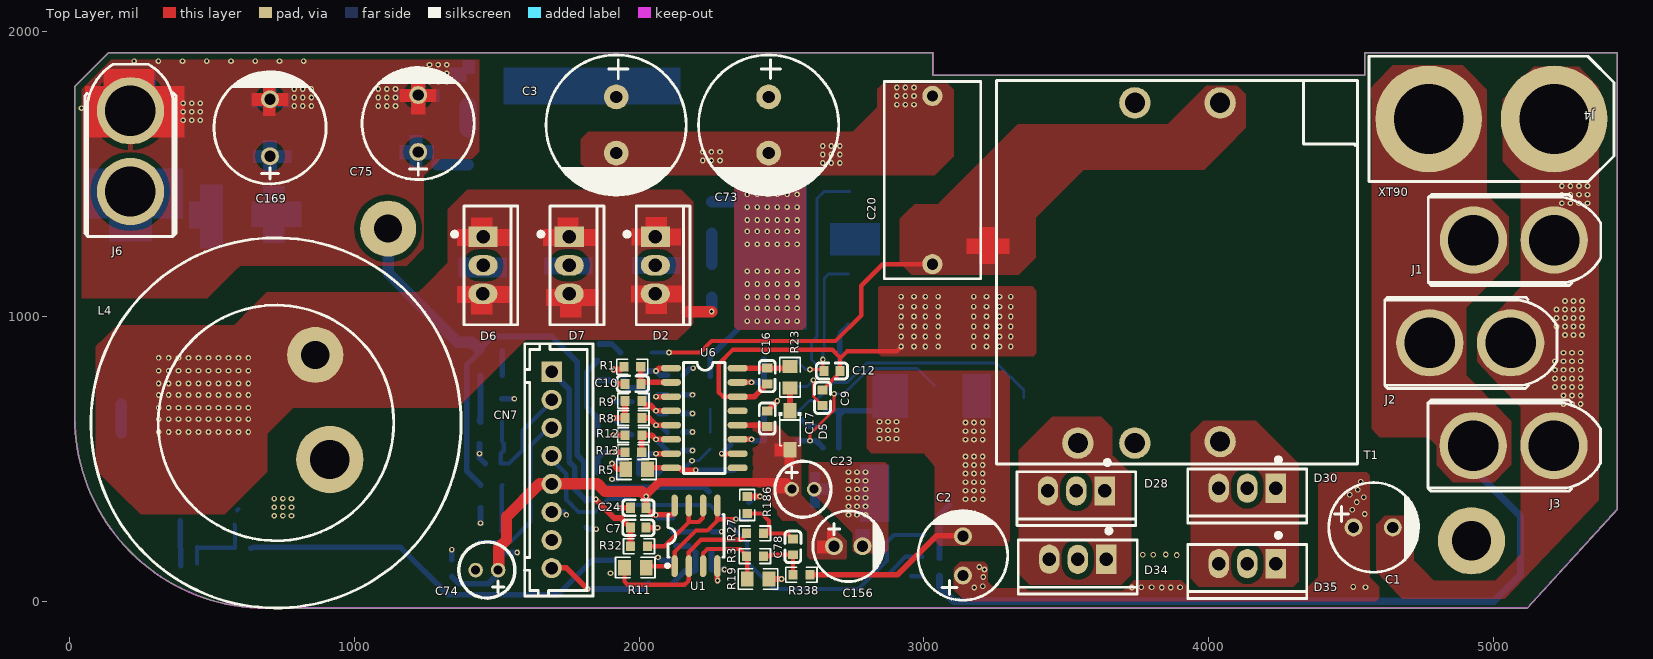
[diagram p0: Top Layer view]
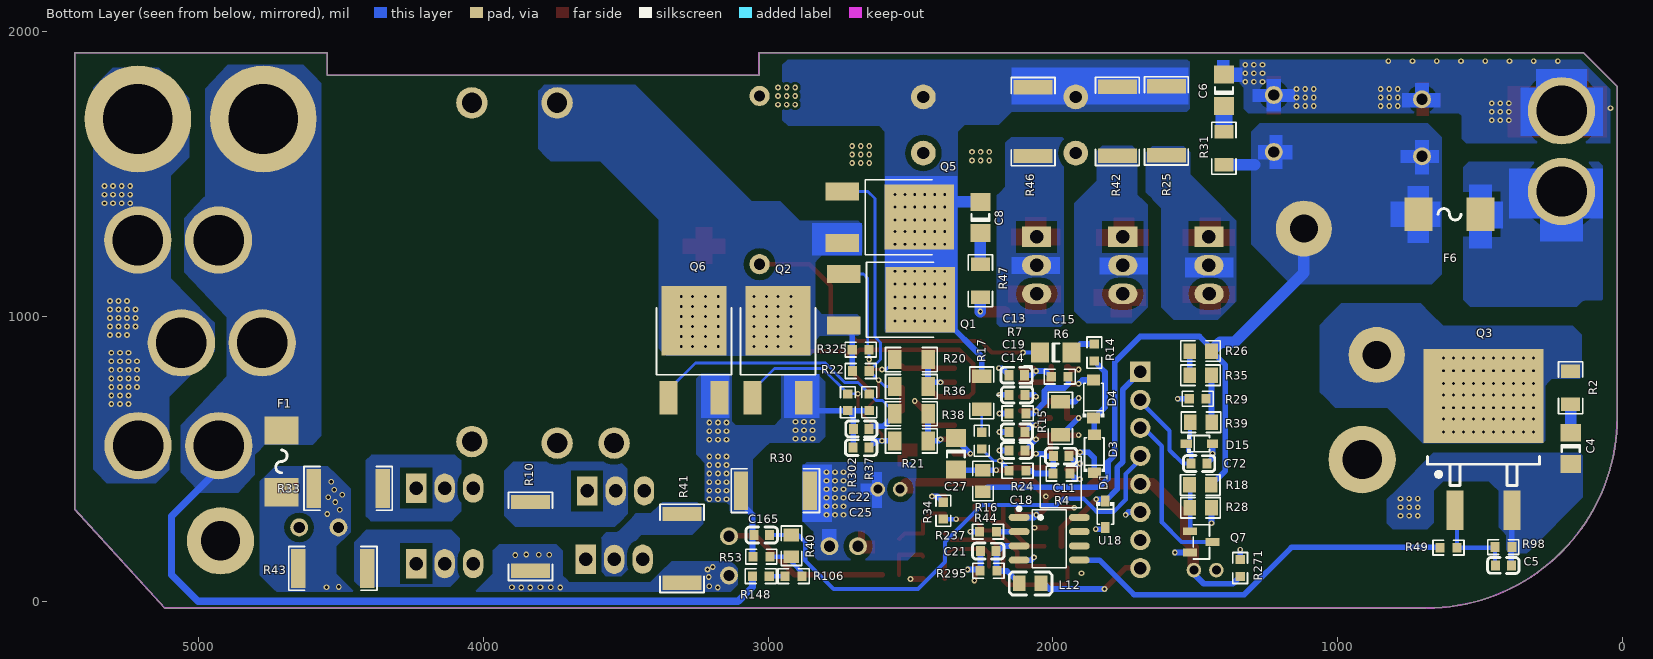
[diagram p1: Bottom Layer view, seen from below]
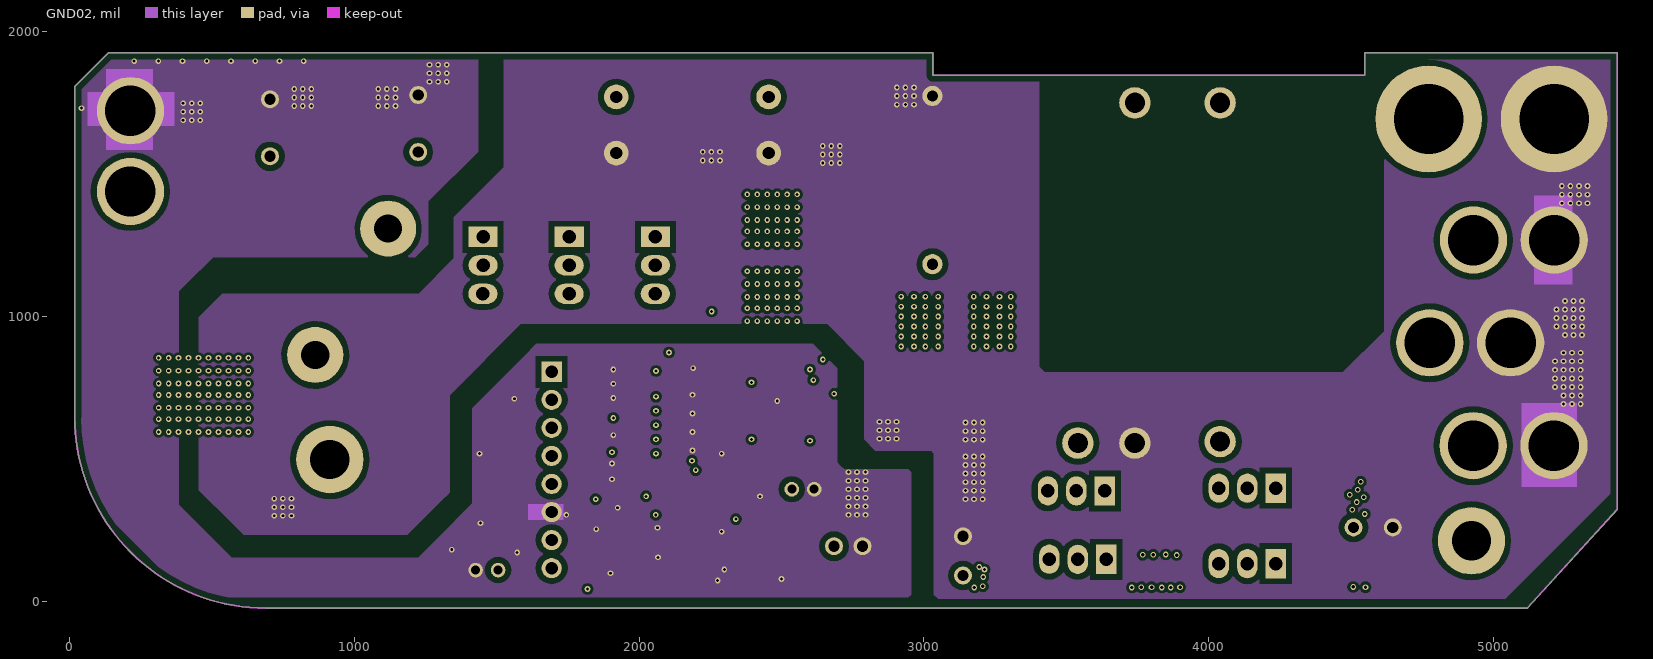
[diagram p2: GND02]
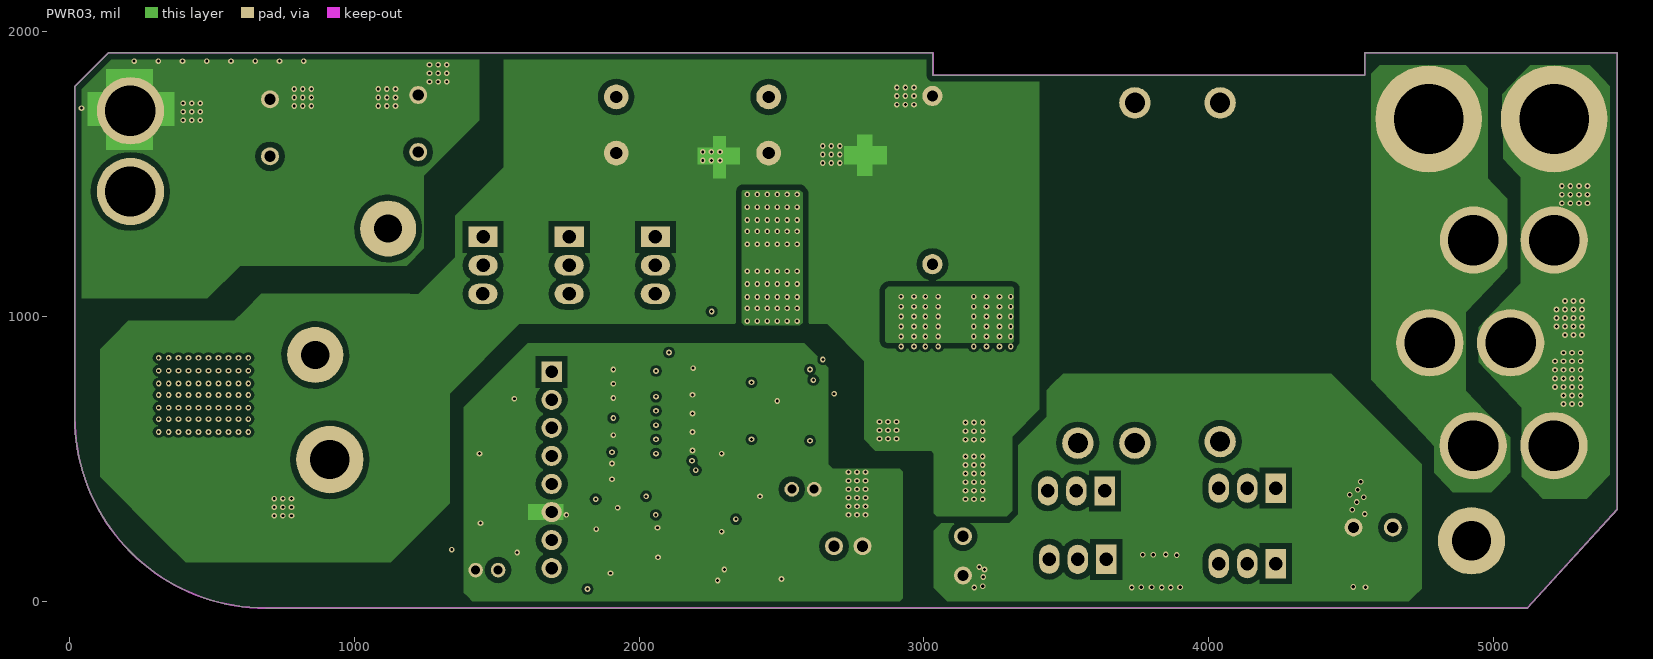
[diagram p3: PWR03]
# Altium PCB MISC84449.PcbDoc (part 1 of 3)
Units mil, origin at the board's own origin, x right, y up, seen from the top; angles counter-clockwise.
Board outline 5413.39 x 1948.82 mil, 4 copper layers (Top Layer, GND02, PWR03, Bottom Layer); 124 components, 66 nets, 298 pads, 442 vias.

## Layer stack, top to bottom (the 12.6 mil dielectric is the usual default, probably not edited)
Top Layer: signal copper 1.4
Dielectric: core 12.6, FR-4, Dk 4.8
GND02: signal copper 1.4
Dielectric: prepreg 12.6, FR-4, Dk 4.8
PWR03: signal copper 1.4
Dielectric: core 12.6, FR-4, Dk 4.8
Bottom Layer: signal copper 1.4

## Board outline
689.14,-22.12 cw(c689.14,647.18) 19.85,647.18 19.85,1808.59 137.96,1926.7 3031.66,1926.7 3031.66,1847.96 4547,1847.96 4547,1926.7 5433.24,1926.7 5433.24,324.34 5118.28,-22.12

## Design rules (kind name [scope] priority, off if disabled: settings)
Clearance 40 [InNetClass('40')] p1 off: gap=30
Clearance Clearance_via [isvia vs inpoly] p2: gap=10
Clearance [InPolygon] p3: gap=20
Clearance all [All] p4: gap=8
ComponentClearance [All] p1 off: gap=10 collisioncheckmode=3 verticalgap=10 showdistances=FALSE
FabricationTestPointUsage TestPointUsage [All] p1: valid=0 allowmultiple=FALSE
FabricationTestpoint Testpoint [(IsPad And (OnTopLayer Or OnBottomLayer))] p1: side=3 testpointundercomponent=TRUE minsize=40 maxsize=100 preferedsize=60 minholesize=0 maxholesize=40 preferedholesize=32 testpointgrid=1 allowsidetop=TRUE allowsidebottom=TRUE usegrid=TRUE gridtolerance=0.01
Height [All] p1 off: minheight=0 maxheight=1000 prefheight=500
HoleSize [All] p1 off: absolutevalues=TRUE maxlimit=100 minlimit=1 maxpercent=80.000 minpercent=20.000
HoleToHoleClearance [All] p1 off: gap=10 allowstackedmicrovias=TRUE
LayerPairs [All] p1 off: enforce=TRUE
MinimumSolderMaskSliver [All] p1 off: minsoldermaskwidth=10
NetAntennae [All] p1: netantennaetolerance=1
PlaneClearance [All] p1: clearance=12
PlaneConnect [All] p1: planeconnectstyle=Relief reliefexpansion=8 reliefentries=4 reliefconductorwidth=10 reliefairgap=10
PolygonConnect PolygonConnect_1 [ISVIA] p1: connectstyle=Direct reliefconductorwidth=10 reliefentries=4 polygonreliefangle="90 Angle"
PolygonConnect [All] p2: connectstyle=Direct reliefconductorwidth=35 reliefentries=4 polygonreliefangle="90 Angle"
RoutingVias [All] p1: holewidth=10 width=20 viastyle="Through Hole" minholewidth=10 minwidth=20 maxholewidth=12 maxwidth=20
SilkToSilkClearance [All] p1 off: silktosilkclearance=10
SilkscreenOverComponentPads [IsPad] p1 off: minsilkscreentomaskgap=10
SolderMaskExpansion [All] p1: expansion=2.5
Width [All] p1: maxlimit=500 minlimit=10 preferedwidth=10
15 further rules are at their usual default settings.

## Components (designator, comment, footprint, x,y, rotation, side; value= is the part's Value field where it differs from the comment)
C1 "390uF" CAP-TH_BD8.0-P3.50-D0.6-FD 4577.65,261.02 r0 top
C2 "390uF" CAP-TH_BD8.0-P3.50-D0.6-FD 3136.98,161.85 r90 top
C3 "560uF" CAP-TH_BD12.5-P5.00-D0.6-FD 1919.99,1673.43 r270 top
C4 "2.2nF" C1206 183,538.12 r270 bottom
C5 "2.2nF" C0603 419.08,127.64 r180 bottom
C6 "2.2nF" C1206 1400,1795.12 r90 bottom
C7 "1nF" C0603 1997.44,260 r180 top
C8 "2.2nF" C1206 2255,1348.68 r90 bottom
C9 "2.2nF" C0603 2644.36,715.92 r90 top
C10 "220nF" C0603 1978.64,765 r0 top
C11 "1uF" C0603 1971.32,511.12 r180 bottom
C12 "2.2nF" C0603 2677.64,810.08 r0 top
C13 "2.2uF" C0603 2127.44,795 r180 bottom
C14 "1nF" C0603 2126.32,596.12 r180 bottom
C15 "NC" C1206 1990,875 r180 bottom
C16 "100nF" C0603 2450,792.44 r90 top
C17 "100nF" C0603 2450,642.56 r270 top
C18 "470pF" C0603 2126.32,531.12 r180 bottom
C19 "1nF" C0603 2126.32,726.12 r0 bottom
C20 "680nF" CAP-TH_L17.5-W8.5-P15.00-D0.8 3030,1480 r90 top
C21 "220pF" C0603 2227.08,177.64 r180 bottom
C22 "2.2nF" C0603 2672.64,606.92 r0 bottom
C23 "22uF" CAP-TH_BD5.0-P2.00-D0.8-FD 2575.63,395 r0 top
C24 "100nF" C0603 1997.44,330 r180 top
C25 "2.2nF" C0603 2673.64,540.92 r0 bottom
C27 "10nF" C1206 2340.92,519.36 r270 bottom
C72 "100nF" C0603 1487.44,485 r0 bottom
C73 "560uF" CAP-TH_BD12.5-P5.00-D0.6-FD 2454.99,1673.43 r270 top locked
C74 "22uF" CAP-TH_BD5.0-P2.00-D0.8-FD 1466.08,111.36 r180 top
C75 "390uF" CAP-TH_BD10.0-P5.00-D1.0-FD 1225,1680 r90 top
C78 "100nF" C0603 2540,192.56 r270 top
C156 "220uF" CAP-TH_BD6.3-P2.50-D1.0-FD 2735,195 r0 top
C165 "100nF" C0603 3022,234 r180 bottom
C169 "390uF" CAP-TH_BD10.0-P5.00-D1.0-FD 705,1665 r90 top
CN7 "HX25003-8A" CONN-TH_8P-P2.50_HX25003-8A 1718.92,462.64 r90 top
D1 "MM3Z3V3_C123917" SOD-323_L1.8-W1.3-LS2.5-RD 1816,307.16 r270 bottom
D2 "SBD20C200T" TO-220-3_L10.0-W4.5-P2.54-L 2067.14,1181 r270 top
D3 "1N4148W_C388533" SOD-123_L2.8-W1.8-LS3.7-RD 1855,520 r90 bottom
D4 "1N4148W_C388533" SOD-123_L2.8-W1.8-LS3.7-RD 1858,711.63 r90 bottom
D5 "FR107_C2760867" SOD-123FL_L2.7-W1.8-LS3.8-RD 2530,601.7 r270 top
D6 "SBD20C200T" TO-220-3_L10.0-W4.5-P2.54-L 1462.14,1181 r270 top
D7 "SBD20C200T" TO-220-3_L10.0-W4.5-P2.54-L 1764.64,1181 r270 top
D15 "MM3Z3V3_C123917" SOD-323_L1.8-W1.3-LS2.5-RD 1486.16,555 r180 bottom
D28 "SBT40100VCT" TO-220-3_L10.0-W4.5-P2.54-L 3535,379.53 r180 top
D30 "SBT40100VCT" TO-220-3_L10.0-W4.5-P2.54-L 4135,389.14 r180 top
D34 "SBT40100VCT" TO-220-3_L10.0-W4.5-P2.54-L 3540,139.53 r180 top
D35 "SBT40100VCT" TO-220-3_L10.0-W4.5-P2.54-L 4135,124.14 r180 top
F1 "20A/200V" FUSE-SMD_L6.1-W2.5 4708.08,492.64 r90 bottom
F6 "10A/200V" FUSE-SMD_L6.1-W2.5 608.27,1360 r0 bottom
J1 "XT60" CONN-TH_XT60UPB-F 5072.92,1269.64 r180 top
J2 "XT60" CONN-TH_XT60UPB-F 4920,909 r180 top
J3 "XT60" CONN-TH_XT60UPB-F 5072,548 r180 top
J4 "XT60HOLE" XT90N 4991.8,1694.54 r180 top
J6 "6A" CONN-TH_XT60UPB-F 215,1584.23 r270 top
L4 "330uH" 200W-TMS330060A 785,730 r60 top locked
L12 "BLM21PG300SN1D" L0805 2079.92,64.36 r0 bottom
Q1 "NCEP1520K" TO-252-2_L6.6-W6.1-P4.57-LS9.9-BR-CW 2575,1060 r0 bottom
Q2 "NCEP1520K" TO-252-2_L6.6-W6.1-P4.57-LS9.9-BR-CW 2965,876 r270 bottom
Q3 "CRSS042N10N" TO-263-3_L10.2-W10.7-P5.08-LS16.2-TL 488.99,570.04 r90 bottom locked
Q5 "NCEP1520K" TO-252-2_L6.6-W6.1-P4.57-LS9.9-BR-CW 2579.78,1350 r0 bottom
Q6 "NCEP1520K" TO-252-2_L6.6-W6.1-P4.57-LS9.9-BR-CW 3260,876.22 r270 bottom
Q7 "MMBT3904" SOT-23-3_L2.9-W1.3-P1.90-LS2.4-BR 1479.37,210 r0 bottom
R1 "1.5M" R0603 1976.54,825 r0 top
R2 "" R1206 172.49,782.73 r270 bottom
R3 "" R0603 2406.71,160 r0 top
R4 "" R0603 1969.65,450 r0 bottom
R5 "" R0805 1980.34,465 r0 top
R6 "3K" R0603 1976.54,790 r0 bottom
R7 "" R0603 2124.22,661.12 r0 bottom
R8 "" R0603 1980.65,645 r0 top
R9 "3.65K" R0603 1980.34,705 r180 top
R10 "" R2512 3834,229.28 r270 bottom
R11 "100K" R0805 1998.29,120 r180 top
R12 "" R0603 1980.34,585 r0 top
R13 "" R0603 1980,525 r0 top
R14 "" R0603 1855,874.65 r270 bottom
R15 "10K" R1206 1984.38,612.83 r90 bottom
R16 "" R0603 2250,565.35 r270 bottom
R17 "" R1206 2239.49,764.73 r270 bottom
R18 "100K" R0805 1494.37,410 r180 bottom
R19 "100K" R0805 2406.71,80 r0 top
R20 "10" R1206 2465.27,839.49 r0 bottom
R21 "10" R1206 2465.27,554.49 r0 bottom
R22 "30K" R0603 2674.65,810 r0 bottom
R23 "" R0805 2530,799.37 r270 top
R24 "" R0603 2124.37,460 r180 bottom
R25 "" R2512 1602,1688.28 r90 bottom
R26 "100K" R0805 1493.29,880 r180 bottom
R27 "" R0603 2406.71,240 r0 top
R28 "" R0805 1470.63,330 r0 bottom
R29 "" R0603 1492.05,712.5 r180 bottom
R30 "" R2512 2974.28,390 r0 bottom
R31 "" R1206 1410.51,1560.27 r90 bottom
R32 "1K" R0603 2000,195 r180 top
R33 "" R2512 4473.72,398 r0 bottom
R34 "1K" R0603 2385,319.65 r90 bottom
R35 "0" R0805 1470.63,795 r0 bottom
R36 "10" R1206 2465.27,744.49 r0 bottom
R37 "30K" R0603 2645,700.35 r270 bottom
R38 "10" R1206 2465.27,649.49 r0 bottom
R39 "" R0805 1492.05,630 r180 bottom
R40 "" R0805 2918,185 r90 bottom
R41 "" R2512 3302,187.28 r270 bottom
R42 "" R2512 1774,1686.28 r90 bottom
R43 "" R2512 4527.72,117 r0 bottom
R44 "" R0805 2245.92,435.36 r270 bottom
R46 "" R2512 2070,1685.28 r90 bottom
R47 "" R1206 2265.51,1095.27 r90 bottom
R49 "10" R0603 611.65,190 r0 bottom
R53 "30K" R0603 3023.71,158.29 r180 bottom
R98 "30K" R0603 419.34,192 r0 bottom
R106 "30K" R0603 2910.34,90 r0 bottom
R148 "" R0603 3025.65,90 r0 bottom
R186 "1" R0603 2380,339.65 r90 top
R237 "" R0603 2228.36,246.08 r180 bottom
R271 "" R0603 1343.01,118.36 r270 bottom
R295 "NC" R0603 2226.64,108.92 r0 bottom
R302 "30K" R0603 2720,700.35 r270 bottom
R325 "30K" R0603 2675,885 r0 bottom
R338 "1" R0603 2570,95 r0 top
T1 "" "PQ3230 3:2:2-N" 3790,1154 r180 top
U1 "EG358" SOIC-8_L5.0-W4.0-P1.27-LS6.0-BL 2226.98,188.89 r0 top
U6 "EG6599" SO-16_L10.0-W4.0-P1.27-LS6.2-BL 2221.48,645.06 r270 top
U18 "EG3113" SOP-8_L4.9-W3.9-P1.27-LS6.0-BL 2013.36,221.08 r270 bottom

## Footprints (in the part's own frame and the unit in brackets; to place one, negate y for a bottom-side part, rotate by r counter-clockwise, add the part's x,y. Pads: shape width x height; smd on the part's side, far side on the other; paste and mask are expansions set on the pad)
200W-TMS330060A [mm]
  round 5 hole 2.5: 1(17,0) 2(4,0)
  silkscreen extent -19.5,-16.5 13.5,16.5
C0603 [mm]
  rect 0.8x0.9 smd: 1(-0.7,0) 2(0.7,0)
  silkscreen extent -1.41,-0.71 1.39,0.72
C1206 [mm] "Chip Capacitor; Body 3.2 x 1.6 mm (LxW typ)"
  rect 1.6x1.8 smd: 1(-1.4,0) 2(1.4,0)
  silkscreen extent -0.3,-0.8 0.3,0.8
CAP-TH_BD5.0-P2.00-D0.8-FD [mm]
  round 1.3 hole 0.8: 1(-1,0) 2(1,0)
  silkscreen extent -2.5,-2.5 2.5,2.5
CAP-TH_BD6.3-P2.50-D1.0-FD [mm]
  round 1.6 hole 1: 1(-1.28,0) 2(1.26,0)
  silkscreen extent -3.16,-3.15 3.17,3.15
CAP-TH_BD8.0-P3.50-D0.6-FD [mm]
  round 1.6 hole 1: 1(-1.769,-0.001) 2(1.731,-0.001)
  silkscreen extent -3.98,-4 4.02,4
CAP-TH_BD10.0-P5.00-D1.0-FD [mm]
  round 1.6 hole 1: 1(-2.578,0) 2(2.502,0)
  silkscreen extent -5.04,-5 5.04,5
CAP-TH_BD12.5-P5.00-D0.6-FD [mm]
  round 2.2 hole 1.1: 1(-2.5,0) 2(2.5,0)
  silkscreen extent -6.25,-6.25 6.26,6.25
CAP-TH_L17.5-W8.5-P15.00-D0.8 [mm]
  round 1.8 hole 1: 1(-7.5,0) 2(7.5,0)
  silkscreen extent -8.8,-4.3 8.8,4.3
CONN-TH_8P-P2.50_HX25003-8A [mm]
  rect 1.8x1.8 hole 1.1: 1(8.75,0.646)
  round 1.8 hole 1.1: 2(6.25,0.646) 3(3.75,0.646) 4(1.25,0.646) 5(-1.25,0.646) 6(-3.75,0.646) 7(-6.25,0.646) 8(-8.75,0.646)
  silkscreen extent -11.25,-3.05 11.25,3.05
CONN-TH_XT60UPB-F [mm]
  round 6 hole 4.5: 1(3.663,0) 2(-3.536,0)
  silkscreen extent -7.68,-4.06 7.68,4.06
FUSE-SMD_L6.1-W2.5 [mm]
  rect 2.5x3 smd: 1(-2.75,0) 2(2.75,0)
  silkscreen extent -1.02,-0.51 1.02,0.51
L0805 [mil]
  rect 44.59x54.21 smd: 1(-38.05,0) 2(38.04,0)
  silkscreen extent -77,-40 73,40
"PQ3230 3:2:2-N" [mm]
  round 2.8 hole 1.8: 3(-6.342,-15.17) 4(1.258,-15.17) 8(6.342,15.17) 9(1.262,15.17) 10(-6.342,15.03)
  silkscreen extent -18.59,-17.17 13.61,17.03
R0603 [mil]
  rect 31.75x34.02 smd: 1(-29.65,0) 2(29.65,0)
  silkscreen extent -55,-26 55,26
R0805 [mil]
  rect 44.59x54.21 smd: 1(-26.71,0) 2(49.37,0)
  silkscreen extent -58,-36 81,36
R1206 [mil]
  rect 47.54x66.97 smd: 1(-26.71,-10.51) 2(89.73,-10.51)
  silkscreen extent -59,-53 122,32
R2512 [mil]
  rect 50.49x136.06 smd: 1(-120.72,0) 2(120.72,0)
  silkscreen extent -155,-77 155,77
SO-16_L10.0-W4.0-P1.27-LS6.2-BL [mm]
  oval 0.6x1.8 smd: 1(-4.444,-2.776) 2(-3.174,-2.776) 3(-1.904,-2.776) 4(-0.634,-2.776) 5(0.636,-2.776) 6(1.906,-2.776) 7(3.176,-2.776) 8(4.446,-2.776) 9(4.446,3.168) 10(3.176,3.168) 11(1.906,3.168) 12(0.636,3.168) 13(-0.634,3.168) 14(-1.904,3.168) 15(-3.174,3.168) 16(-4.444,3.168)
  silkscreen extent -4.95,-1.65 4.95,2.05
SOD-123_L2.8-W1.8-LS3.7-RD [mm]
  rect 0.95x1.15 smd: 1(-1.693,0) 2(1.693,0)
  silkscreen extent -1.63,-0.94 1.41,0.94
SOD-123FL_L2.7-W1.8-LS3.8-RD [mm]
  rect 1.4x1.2 smd: 1(-1.735,0) 2(1.735,0)
  silkscreen extent -1.6,-1 1.38,1
SOD-323_L1.8-W1.3-LS2.5-RD [mm]
  rect 1x0.75 smd: 1(-1.173,0) 2(1.173,0)
  silkscreen extent -1.08,-0.8 0.9,0.8
SOIC-8_L5.0-W4.0-P1.27-LS6.0-BL [mil]
  oval 22.38x76.78 smd: 1(-101.98,-63.89) 2(-51.98,-63.89) 3(-1.98,-63.89) 4(48.02,-63.89) 5(48.02,149.11) 6(-1.98,149.11) 7(-51.98,149.11) 8(-101.98,149.11)
  silkscreen extent -133,-68 71,118
SOP-8_L4.9-W3.9-P1.27-LS6.0-BL [mm]
  oval 0.63x1.865 smd: 1(-1.905,-2.682) 2(-0.635,-2.682) 3(0.635,-2.682) 4(1.905,-2.682) 5(1.905,2.682) 6(0.635,2.682) 7(-0.635,2.682) 8(-1.905,2.682)
  silkscreen extent -2.82,-2.83 2.58,1.52
SOT-23-3_L2.9-W1.3-P1.90-LS2.4-BR [mm]
  rect 1.25x0.7 smd: 1(1,-0.95) 2(1,0.95) 3(-1,0)
  silkscreen extent -0.73,-1.53 0.73,1.53
TO-220-3_L10.0-W4.5-P2.54-L [mm]
  rect 1.8x2.6 hole 1.2: 1(-2.54,-0.241)
  oval 1.8x2.6 hole 1.2: 2(0,-0.241) 3(2.54,-0.251)
  silkscreen extent -5.3,-2.98 5.3,2.85
TO-252-2_L6.6-W6.1-P4.57-LS9.9-BR-CW [mm]
  rect 3x1.6 smd: 1(4.06,-2.29) 3(4.06,2.29)
  rect 6.2x5.8 smd: 2(-2.788,0)
  silkscreen extent -3.95,-3.35 2.02,3.35
TO-263-3_L10.2-W10.7-P5.08-LS16.2-TL [mm]
  rect 3.504x1.5 smd: 1(-6.325,2.54) 3(-6.325,-2.54)
  rect 8.38x10.7 smd: 2(3.888,0)
  silkscreen extent -4.11,-5 -1.51,5
XT90N [mm]
  round 9.5 hole 6.2: 1(5.588,0) 2(-5.588,0)
  silkscreen extent -10.92,-5.59 10.92,5.59

## Free pads (board coordinates)
  round 236.22 hole 137.8: 0(915,499) 0(4922,214)

## Via types
v1: diameter 20, hole 10, Top Layer to Bottom Layer, tented both sides, 231 vias
v2: diameter 20, hole 10, Top Layer to Bottom Layer, 187 vias
v3: diameter 20, hole 12, Top Layer to Bottom Layer, 24 vias

## Nets (pads, with @x,y where several pads share a name; then routed paths per layer and width w, separated by ;. In a path a pad name is that pad's centre, name@x,y a point inside that pad or via, vN(x,y) a via of type N, cw(c..) or ccw(c..) an arc to the next point about the centre after c; other vN are vias at no path point)
+12V: C17.2 C23.1 C24.1 C74.1 C156.1 CN7.5 D5.2 R271.2 U1.8 U6.12 U18.1 | length 1841.9
  Top Layer w20: v1(2025,370) C24.1@2025,330 v2@2050,305 ; v2(2059,305) 2115,305 2125,315 U1.8@2125,338 U1.8@2125,355 ; U6.12@2346.19,620 C17.2@2450,620
  Top Layer w30: v1@2020.5,374.5 v1(2025,370) 2025,375 2070,420 2517,420 C23.1@2532,405
  Top Layer w40: C74.1@1508,122.36 1508,190 1535,217 1535,298 1651,414 1854,414 1881,387 2009,387 v1@2021,375
  Bottom Layer w20: R271.2@1343.01,88.71 1368.72,63 1471.09,63 C74.1@1518.45,110.36 ; v2@2057,306 2059.48,303.52 2060.48,303.52 2064.44,299.56 2064.44,298.56 2066.92,296.08 U18.1@2118.97,296.08
B+: F1.2 J1.1 J2.1 J3.1 J4.1 R148.2 | length 2549.8
  Bottom Layer w25: R148.2@3055,91 3055,52 3105,2 5001,2 5094,95 5094,300 4955,439 J3.1@4955,450
BAT-: C1.2 C2.2 C3.2 C4.2 C5.2 C20.2 C22.2 C25.2 C73.2 C165.1 J1.2 J2.2 J3.2 J4.2 Q2.3 Q3.3 Q6.3 R30.2 R37.2 R53.1 R98.1 R302.2 R338.2 T1.9 | length 1273.4
  Top Layer w20: R338.2@2599.65,95 2907,95 3044,232 C2.2@3129,232
  Bottom Layer w20: R98.1@389.69,192 Q3.3@389.69,283.31 ; C5.2@391.52,127.64 R98.1@391.52,184.52 ; R37.2@2655,670.69 R302.2@2720,670.69 Q2.3@2859.31,670.69 ; C25.2@2701.19,540.92 2701.19,653.19 R302.2@2716,668 ; C165.1@3054.55,222 3054.55,305.56 R30.2@3090,341 ; R53.1@3054.65,153 C165.1@3054.65,220.9
  other v1: 720,302 750,302 780,302 720,332 750,332 780,332 3146,360 3176,360 3206,360 720,362 750,362 780,362 3146,390 3176,390 3206,390 3146,420 3176,420 3206,420 3146,450 3176,450 3206,450 3146,480 3176,480 3206,480 3146,510 3176,510 3206,510 3146,569 3176,569 3206,569 2844,572 2874,572 2904,572 3146,599 3176,599 3206,599 2844,602 2874,602 2904,602 3146,629 3176,629 3206,629 2844,632 2874,632 2904,632 5245,694 5275,694 5305,694 5245,724 5275,724 5305,724 5215,754 5245,754 5275,754 5305,754 5215,784 5245,784 5275,784 5305,784 5215,814 5245,814 5275,814 5305,814 5215,844 5245,844 5275,844 5305,844 5245,874 5275,874 5305,874 5250,936 5280,936 5310,936 5220,966 5250,966 5280,966 5310,966 5220,996 5250,996 5280,996 5310,996 5220,1026 5250,1026 5280,1026 5310,1026 5250,1056 5280,1056 5310,1056 5239,1399 5269,1399 5299,1399 5329,1399 5239,1429 5269,1429 5299,1429 5329,1429 5239,1459 5269,1459 5299,1459 5329,1459 2645,1540 2675,1540 2705,1540 2224,1549 2254,1549 2284,1549 2645,1570 2675,1570 2705,1570 2224,1579 2254,1579 2284,1579 2645,1600 2675,1600 2705,1600 2905,1745 2935,1745 2965,1745 2905,1775 2935,1775 2965,1775 2905,1805 2935,1805 2965,1805
BAT-V: C165.2 CN7.4 R40.2 | length 1737.2
  Bottom Layer w15: CN7.4@1701,492 1744.42,448.58 1744.42,358.58 1788,315 1846,315 1893,362 1964,362 1986,340 2249,340 2379,210 2379,140 2474,45 2770,45 2870,145 2870,210 2894.37,234.37 C165.2@3001,234.37 ; CN7.4@1703,498 CN7.4@1705,496